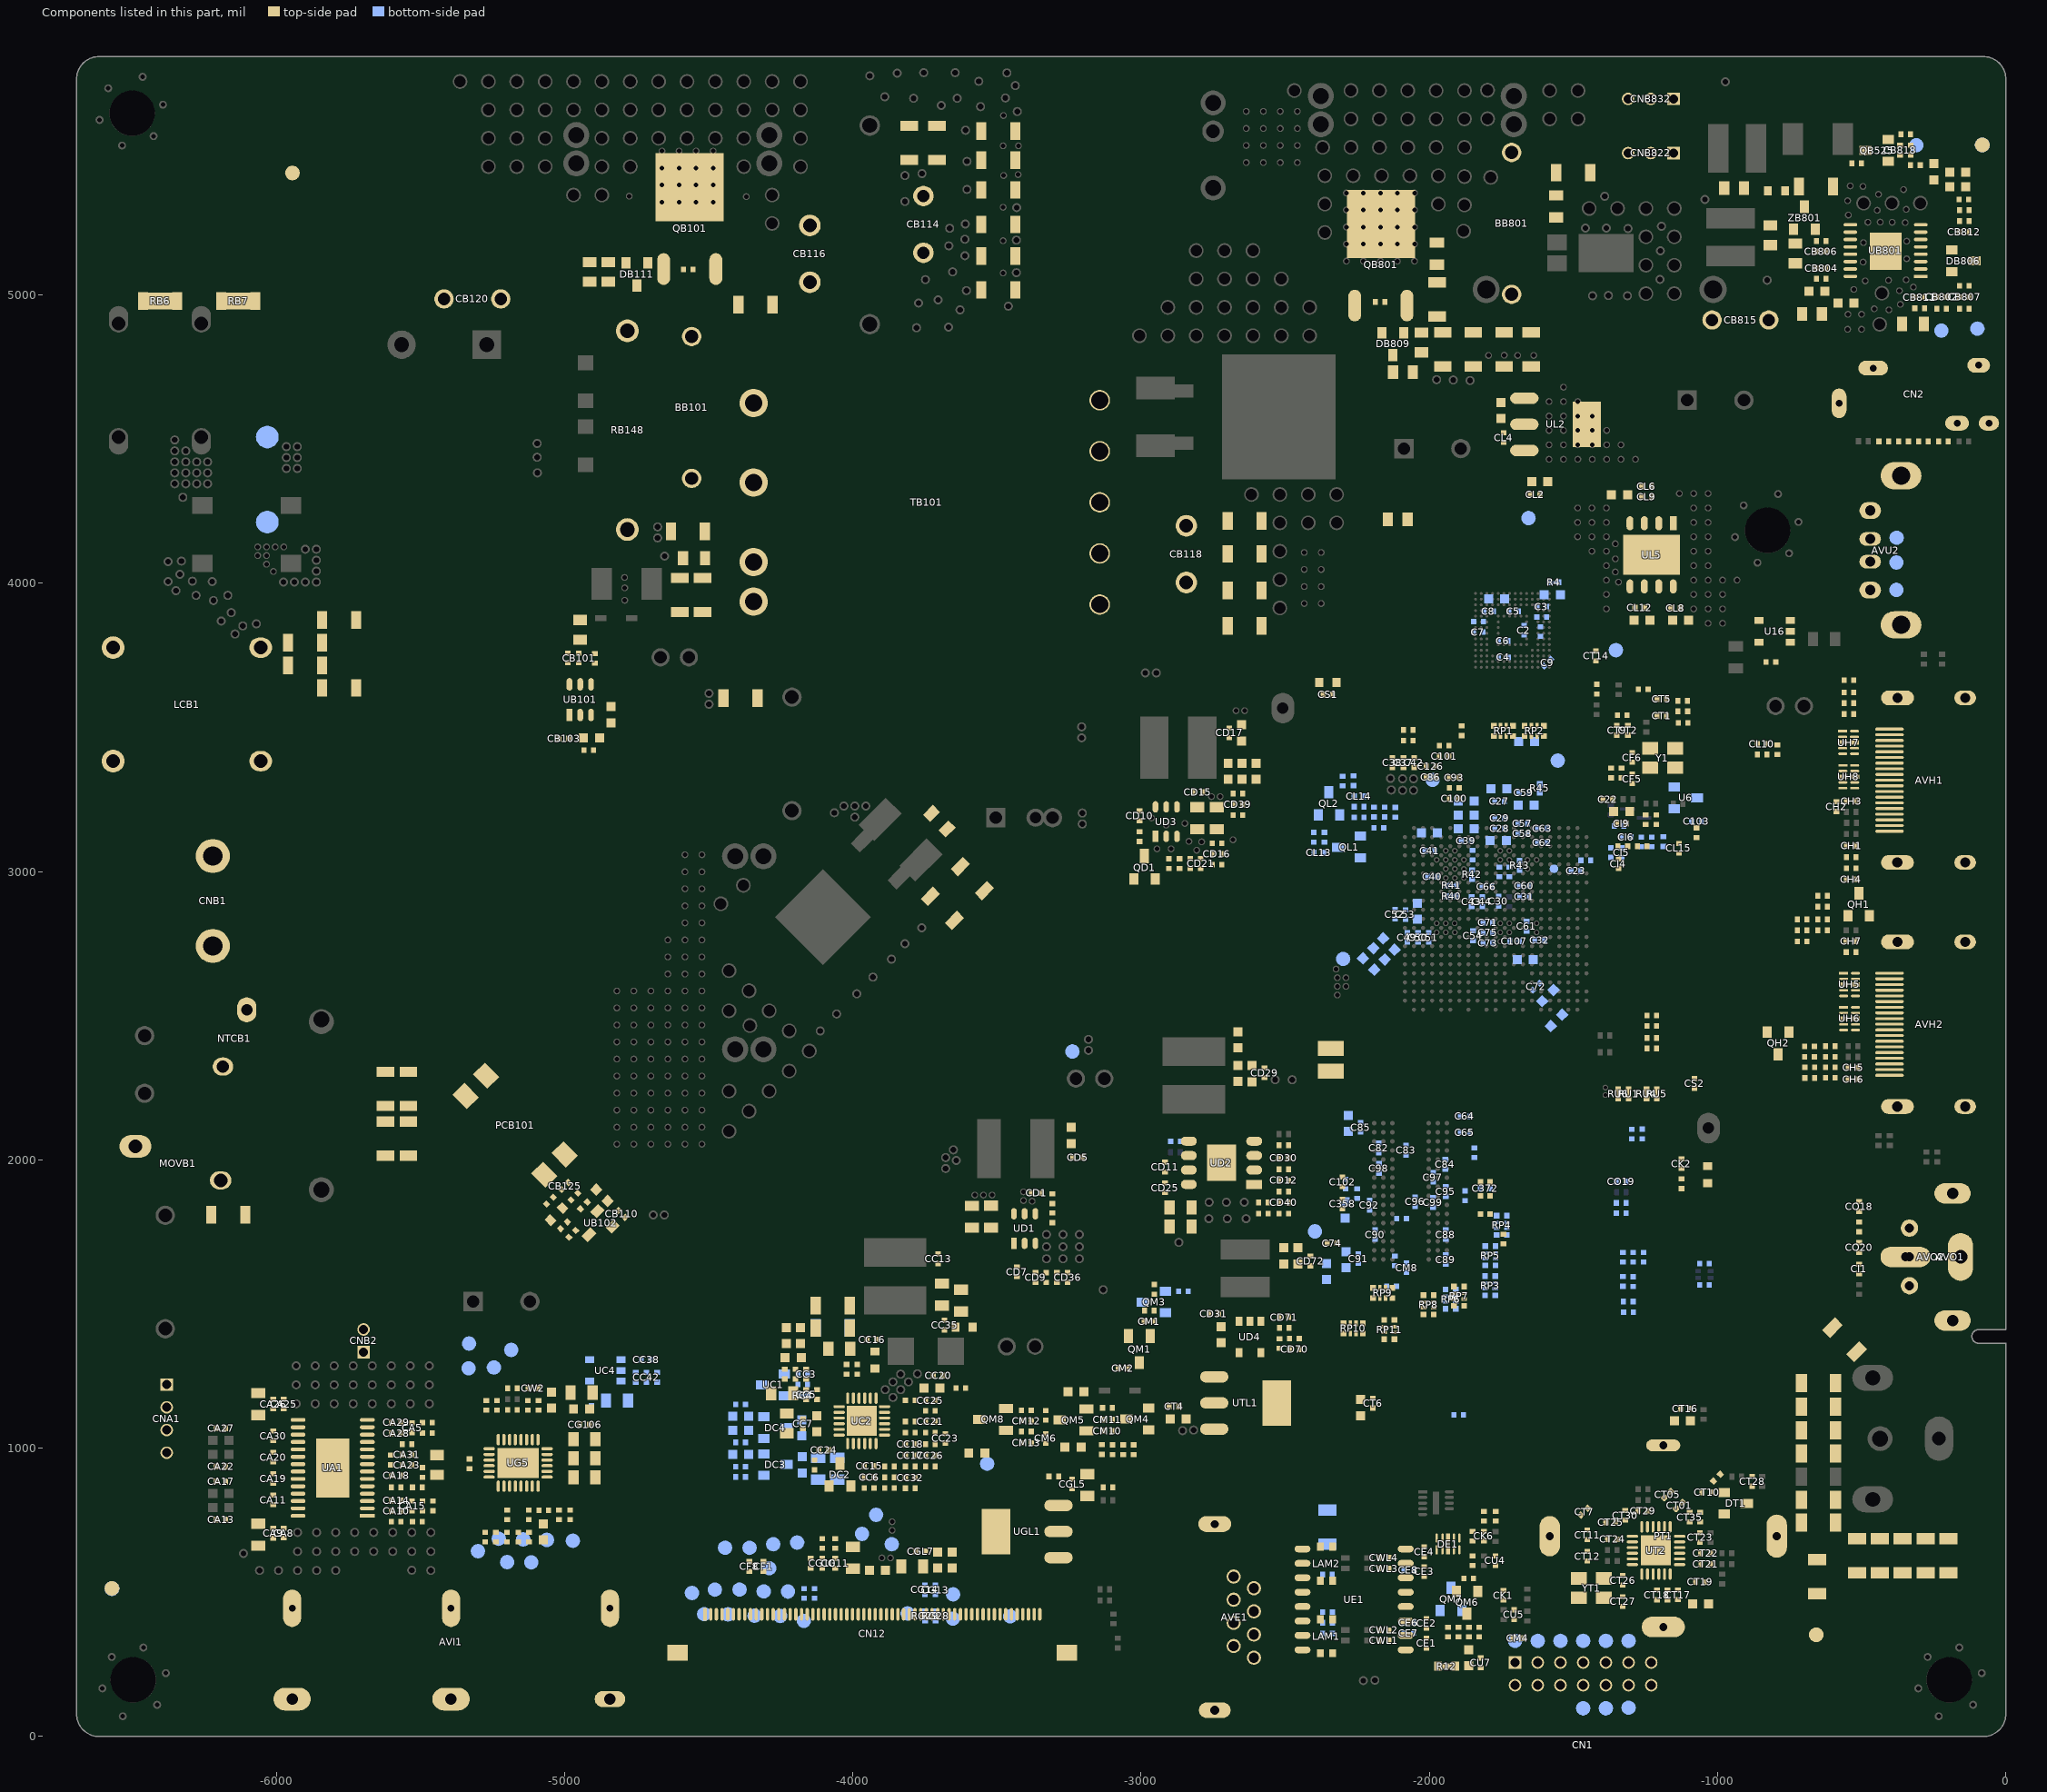
[diagram p0: the components of this part, seen from the top]
# Altium PCB MISC84395.PcbDoc (part 6 of 26)
Units mil, origin at the board's own origin, x right, y up, seen from the top; angles counter-clockwise.
Board outline 6692.91 x 5826.77 mil, 2 copper layers (TopLayer, BottomLayer), stack 61.855 mil thick; 951 components, 565 nets, 4374 pads, 1804 vias.
Unrouted connection lines stored in the file: 1.

## Footprints (in the part's own frame and the unit in brackets; to place one, negate y for a bottom-side part, rotate by r counter-clockwise, add the part's x,y. Pads: shape width x height; smd on the part's side, far side on the other; paste and mask are expansions set on the pad) (continued)
L/LC4/3.2*1.6 [mil] "sunlord,DCM321620F2SF-600T02,17.09.19"
  rect 28x24 smd: 1(59.06,21.65) 2(-59.06,21.65) 3(-59.06,-21.65) 4(59.06,-21.65)
  silkscreen extent -38,-35 99,35, body extent -75,-35 75,35, height 87
L/UU10.5/10*13-2 [mm] "SYUU10.5-L001(协兴电子) 卡扣在侧面"
  oval 1.8x2 hole 1.2: 1(5,-6.5) 4(-5,-6.5)
  round 2 hole 1.2: 2(5,6.5) 3(-5,6.5)
  round 2.2 on Top Overlay: 4(-5,6.5) 4(5,6.5)
  oval 2x2.2 on Top Overlay: 4(-5,-6.5) 4(5,-6.5)
  silkscreen extent -8,-9.25 11.5,9.25, body extent -8,-8.5 9.5,8.5, height 13.8
LB/3.5*6*12.5#1 [mm] "Φ3.5×6.0×0.65mm(编带/秀益达)"
  round 1.7 hole 1.15: 1(-6.25,0) 2(6.25,0)
  round 1.9 on Top Overlay: 35(-6.25,0) 36(6.25,0)
  BottomLayer lines w0.6: 6.185,-0.532 4.05,0 ; -6.185,-0.532 -6.121,-0.516 -4.05,0 ; 6.25,0 4.05,0 ; -6.25,0 -4.05,0 ; 6.185,0.532 4.05,0 ; -6.185,0.532 -6.121,0.516 -5.811,0.439 -4.05,0
  silkscreen extent -5.6,-1.85 5.65,1.85, body extent -6.57,-1.75 6.58,1.75, height 3.5
LB/3.5*6*12.5#2 [mm] "Φ3.5×6.0×0.65mm(编带/秀益达)"
  round 1.7 hole 1.15: 1(-6.25,0) 2(6.25,0)
  round 1.9 on Top Overlay: 35(-6.25,0) 36(6.25,0)
  BottomLayer lines w0.6: 6.185,-0.532 4.05,0 ; -6.185,-0.532 -4.05,0 ; 6.25,0 4.05,0 ; -6.25,0 -4.05,0 ; 6.185,0.532 4.05,0 ; -6.185,0.532 -4.05,0
  silkscreen extent -5.6,-1.85 5.65,1.85, body extent -6.57,-1.75 6.58,1.75, height 3.5
Manufacture_Info [mm]
  round 0.3 on Mech2: 0(0,0)
MARK [mm] "SMD 使用"
  round 1.3 smd paste+0 mask+0.65: 0(0,0)
  TopLayer circle w0.254: c0,0 r1.444
  TopLayer pour cut-out: -1.3,0 -1.201,-0.497 -0.919,-0.919 -0.497,-1.201 0,-1.3 0,-1.3 0.497,-1.201 0.919,-0.919 1.201,-0.497 1.3,0 1.3,0 1.201,0.497 0.919,0.919 0.497,1.201 0,1.3 0,1.3 -0.497,1.201 -0.919,0.919 -1.201,0.497 -1.3,0
Mylar [mil] "180×180×0.4mm-PC-黑色"
NTC(10*5)-V5 [mm] "热敏电阻 SCK152R58MSY  (为勤电子）;161022更新椭圆孔"
  oval 1.6x1.8 hole 1.1: 1(-2.5,1.05)
  oval 1.6x2 on Top Overlay: 2(-2.5,1.05)
  oval 2.2x1.7 hole 1 slot 1.5 at 0 deg: 2(2.5,-1.05)
  oval 2.4x1.9 on Top Overlay: 3(2.5,-1.05)
  silkscreen extent -5.77,-2.5 5.77,2.5, body extent -5.75,-2 5.75,2, height 13.75
OC4-S-1 [mm] "巨路国际；肖特基LTV-817S-TA-B"
  rect 1.5x1.8 smd: 1(-1.27,-4.9) 2(1.27,-4.9) 3(1.27,4.9) 4(-1.27,4.9)
  silkscreen extent -3.17,-5.35 2.55,3.5, body extent -6.95,-6.95 6.95,6.95, height 3.88
OPTICAL-HD-3 [mm] "强生GQ-03-08  通用封装 (TR）  塑胶整体高度11.6mm，中心高度6mm(17.04.28,增加丝印宽度到12.3mm）"
  oval 2x3.4 on Top Overlay: 0(-5.6,4.7) 0(5.6,4.7)
  round 1.778 on Top Overlay: 0(-2.54,8.5) 0(0,8.5) 0(2.54,8.5)
  round 1.524 hole 0.8: 1(-2.54,8.5) 2(0,8.5) 3(2.54,8.5)
  oval 1.8x3.2 hole 1 slot 2.4 at 90 deg: 4(-5.6,4.7) 5(5.6,4.7)
  silkscreen extent -6.15,0 6.15,11.8
PCB_NAME [mm]
  round 0.3 on Mech2: 0(0,0)
PCB_TIME [mm]
  round 0.3 on Mech2: 0(0,0)
PHONE-HD-54 [mm] "CS,PJ-304L-EP(706-0003-0661),中心高度2.5mm，19.03.15"
  oval 1.5x2.3 on Top Overlay: 0(-2.55,4.3)
  oval 1.5x2 on Top Overlay: 0(-2.55,1.5)
  oval 2.8x1.5 on Top Overlay: 0(-0.8,14.7)
  round 1.8 on Keep-Out: 0(0,10.5) 0(0,3.5)
  oval 1.5x2.8 on Top Overlay: 0(2.3,11.7)
  oval 1.5x2.2 on Top Overlay: 0(2.55,2.4)
  oval 1.3x2 hole 0.6 slot 1.3 at 90 deg: 1(2.55,2.4)
  oval 1.3x2.6 hole 0.6 slot 1.9 at 90 deg: 2(2.3,11.7)
  oval 1.3x2.1 hole 0.6 slot 1.4 at 90 deg: 3(-2.55,4.3)
  oval 2.6x1.3 hole 0.6 slot 1.9 at 0 deg: 4(-0.8,14.7)
  oval 1.3x1.8 hole 0.6 slot 1.1 at 90 deg: 5(-2.55,1.5)
  silkscreen extent -3.1,0 3.1,14.95, body extent -3,-2.5 3,14.85, height 5
QFN24/0.5-1 [mm] "MxL601(MAXLINEAR)"
  oval 1x0.26 smd: 1(-2.08,1.25) 2(-2.08,0.75) 3(-2.08,0.25) 4(-2.08,-0.25) 5(-2.08,-0.75) 6(-2.08,-1.25) 13(2.08,-1.25) 14(2.08,-0.75) 15(2.08,-0.25) 16(2.08,0.25) 17(2.08,0.75) 18(2.08,1.25)
  oval 0.26x1 smd: 7(-1.25,-2.08) 8(-0.75,-2.08) 9(-0.25,-2.08) 10(0.25,-2.08) 11(0.75,-2.08) 12(1.25,-2.08) 19(1.25,2.08) 20(0.75,2.08) 21(0.25,2.08) 22(-0.25,2.08) 23(-0.75,2.08) 24(-1.25,2.08)
  rect 2.65x2.65 smd paste-0.6 mask-0.6: 25(0,0)
  TopLayer pour cut-out: -2.08,1.25 -2.08,-1.25 -1.25,-2.08 1.25,-2.08 2.08,-1.25 2.08,1.25 1.25,2.08 -1.25,2.08
  silkscreen extent -3.31,-3.51 3.31,3.46, body extent -2.02,-2.02 2.02,2.02, height 1
QFN24/0.5-5 [mm] "BEKEN ,     BK2433;BQ24196(1mm)"
  oval 1x0.27 smd: 1(-2,1.25) 2(-2,0.75) 3(-2,0.25) 4(-2,-0.25) 5(-2,-0.75) 6(-2,-1.25) 13(2,-1.25) 14(2,-0.75) 15(2,-0.25) 16(2,0.25) 17(2,0.75) 18(2,1.25)
  oval 0.27x1 smd: 7(-1.25,-2) 8(-0.75,-2) 9(-0.25,-2) 10(0.25,-2) 11(0.75,-2) 12(1.25,-2) 19(1.25,2) 20(0.75,2) 21(0.25,2) 22(-0.25,2) 23(-0.75,2) 24(-1.25,2)
  rect 2.667x2.667 smd paste-0.6 mask-0.6: 25(0,0)
  silkscreen extent -3.38,-3.5 3.1,3.5, body extent -2.05,-2.05 2.05,2.05, height 1
QFN28/0.5-5 [mm] "RICHTEK,RT8939GQW,16.12.16"
  oval 1x0.28 smd: 1(-2.05,1.75) 2(-2.05,1.25) 3(-2.05,0.75) 4(-2.05,0.25) 5(-2.05,-0.25) 6(-2.05,-0.75) 7(-2.05,-1.25) 8(-2.05,-1.75) 15(2.05,-1.75) 16(2.05,-1.25) 17(2.05,-0.75) 18(2.05,-0.25) 19(2.05,0.25) 20(2.05,0.75) 21(2.05,1.25) 22(2.05,1.75)
  oct 1x1 on Top Solder paste-0.1 mask+0.102: 2(-0.66,1.25) 2(-0.66,-1.25) 2(-0.66,0) 3(0.66,1.25) 3(0.66,-1.25) 3(0.66,0)
  oct 1x1 on Top Paste paste-0.1 mask+0.102: 2(-0.66,1.25) 2(-0.66,-1.25) 2(-0.66,0) 3(0.66,1.25) 3(0.66,-1.25) 3(0.66,0)
  oval 0.28x1 smd: 9(-1.25,-2.55) 10(-0.75,-2.55) 11(-0.25,-2.55) 12(0.25,-2.55) 13(0.75,-2.55) 14(1.25,-2.55) 23(1.25,2.55) 24(0.75,2.55) 25(0.25,2.55) 26(-0.25,2.55) 27(-0.75,2.55) 28(-1.25,2.55)
  rect 2.65x3.65 smd paste-3 mask-3: EPAD(0,0)
  silkscreen extent -3.63,-3.93 3.43,3.7, body extent -2.05,-2.55 2.05,2.55, height 0.8
R2-H-17.5 [mm] "只适用于2W小型化"
  round 2 hole 1.3: 1(-8.75,0) 2(8.75,0)
  round 2.2 on Top Overlay: 69(-8.75,0) 69(8.75,0)
  BottomLayer lines w0.6: 8.654,0.643 8.562,0.615 6.55,0 ; -8.665,0.606 -8.583,0.583 ; -8.75,0 -8.634,0 -6.55,0 ; 8.75,0 6.55,0 ; 8.665,-0.606 8.583,-0.583 ; -8.654,-0.643 -8.562,-0.615 -6.55,0 ; -8.583,0.583 -8.583,0.583 ; -8.583,0.583 -6.55,0 ; 6.55,0 8.583,-0.583 ; 8.583,-0.583 8.583,-0.583 ; 8.583,-0.583 8.583,-0.583 ; 8.583,-0.583 8.583,-0.583
  silkscreen extent -8,-2.25 8.1,2.25, body extent -9.14,-2.25 9.14,2.25, height 4.5
R0402 [mm] "片式电阻"
  rect 0.45x0.5 smd mask+0.076: 1(-0.425,0) 2(0.425,0)
  silkscreen extent -0.8,-0.4 0.8,0.4, body extent -0.5,-0.25 0.5,0.25, height 0.5
R0402SC#1 [mm]
  rect 0.45x0.5 smd mask+0.076: 1(-0.425,0) 2(0.425,0)
  rect 0.42x0.25 smd paste-0.5 mask-0.5: 3(0,0)
  silkscreen extent -0.8,-0.4 0.8,0.4, body extent -0.5,-0.25 0.5,0.25, height 0.5
R0402SC#2 [mm]
  rect 0.45x0.5 smd mask+0.076: 1(-0.425,0) 2(0.425,0)
  rect 0.42x0.457 smd paste-0.5 mask-0.5: 3(0,0)
  silkscreen extent -0.8,-0.4 0.8,0.4, body extent -0.5,-0.25 0.5,0.25, height 0.5
R0603 [mm] "贴片电阻"
  rect 0.7x0.8 smd mask+0.076: 1(-0.756,0) 2(0.756,0)
  silkscreen extent -1.25,-0.54 1.25,0.54, body extent -0.8,-0.4 0.8,0.4, height 0.8
R0603SC [mm] "贴片电阻"
  rect 0.7x0.8 smd mask+0.076: 1(-0.756,0) 2(0.756,0)
  rect 0.82x0.5 smd paste-0.5 mask-0.5: 3(0,0)
  silkscreen extent -1.25,-0.54 1.25,0.54, body extent -0.8,-0.4 0.8,0.4, height 0.8
R0805 [mm] "贴片电阻"
  rect 0.9x1.2 smd mask+0.076: 1(-0.866,0) 2(0.866,0)
  silkscreen extent -1.47,-0.75 1.47,0.75, body extent -1,-0.62 1,0.63, height 0.5
R1206 [mm] "贴片电阻"
  rect 0.9x1.55 smd mask+0.076: 1(-1.5,0) 2(1.5,0)
  silkscreen extent -2.1,-0.93 2.1,0.93, body extent -1.6,-0.8 1.6,0.8, height 0.55
R1206SC [mm] "贴片电阻"
  rect 0.9x1.55 smd mask+0.076: 1(-1.5,0) 2(1.5,0)
  rect 2.7x1.5 smd paste-2.7 mask-2.7: 3(0,0)
  silkscreen extent -2.1,-0.93 2.1,0.93, body extent -1.6,-0.8 1.6,0.8, height 0.55
RA0402 [mm] "排阻"
  rect 0.5x0.5 smd mask+0.076: 1(-0.45,0.85) 2(0.45,0.85) 7(-0.45,-0.85) 8(0.45,-0.85)
  rect 0.5x0.3 smd mask+0.076: 3(-0.45,0.25) 4(0.45,0.25) 5(-0.45,-0.25) 6(0.45,-0.25)
  silkscreen extent -0.85,-1.27 0.85,1.27, body extent -0.51,-1 0.51,1, height 0.35
RCL0524P [mm] "RCLAMP0524J(19.03.04 优化丝印）"
  rect 0.21x0.8 smd: 1(-1,-0.52)
  oval 0.21x0.8 smd: 2(-0.5,-0.52) 3(0.5,-0.52) 4(1,-0.52) 5(1,0.52) 6(0.5,0.52) 7(-0.5,0.52) 8(-1,0.52)
  rect 0.38x0.8 smd: GND(0,-0.52) GND(0,0.52)
  silkscreen extent -1.4,-2.03 1.4,1.14, body extent -1.25,-0.6 1.25,0.6, height 0.66
RJ45-VD-16 [mm] "YUQIU,RJ170-F08M1BY-B,19.03.16"
  oval 1.6x3.1 on Top Overlay: 0(-8.2,-1.5) 0(8.2,-1.5)
  round 1.45 on Top Overlay: 0(-3.57,-4.95) 0(-2.55,-3.17) 0(-1.53,-4.95) 0(-0.51,-3.17) 0(0.51,-4.95) 0(1.53,-3.17) 0(2.55,-4.95) 0(3.57,-3.17)
  round 1.25 hole 0.9: 1(3.57,-3.17) 2(2.55,-4.95) 3(1.53,-3.17) 4(0.51,-4.95) 5(-0.51,-3.17) 6(-1.53,-4.95) 7(-2.55,-3.17) 8(-3.57,-4.95)
  oval 1.4x2.8 hole 0.8 slot 2.2 at 90 deg: 9(-8.2,-1.5)
  oval 1.4x2.9 hole 0.7 slot 2.2 at 90 deg: 10(8.2,-1.5)
  silkscreen extent -9.05,-5.93 9.05,5.94, body extent -8.85,-5.77 8.85,5.78, height 13
SHIELD(16*20*6) [mm] "屏蔽罩：用于与高频头分离的做法"
  oval 2.1x4.1 on Top Overlay: 0(-8,10) 0(8,10)
  oval 4.1x2.1 on Top Overlay: 0(0,20) 0(0,0)
  oval 3.8x1.8 hole 0.7 slot 2.7 at 0 deg: 1(0,0)
  oval 1.038x3.013 / inner oval 1.8x3.8 / far side oval 1.8x3.8 hole 0.7 slot 2.7 at 90 deg: 2(8,10)
  oval 3.556x1.8 hole 0.7 slot 2.7 at 0 deg: 3(0,20)
  oval 1.8x3.8 hole 0.7 slot 2.7 at 90 deg: 4(-8,10)
  silkscreen extent -9,-1 9,21, body extent -8.57,-0.15 8.57,20.15, height 6
"Silica gel(3*2*2.5)" [mm] "导电硅胶,3×2×2.5mm;15.09.17"
  rect 1.3x2.3 smd: 1(-1,0) 2(1,0)
  silkscreen extent -1.9,-1.4 1.9,1.4
"Silica gel-10" [mil] "硅胶"
  silkscreen extent -118,-197 118,197
"Silica gel-15" [mil] "硅胶"
  silkscreen extent -118,-295 118,295
SIP2*7H/2.0DM-8 [mm] "XFE,JN-2.0-2×7PW-H=5.6-PC=2.5,公座，19.03.13"
  round 0.8 on Mech2: 0(-6,-3.625) 0(-4,-3.625) 0(-4,-5.625) 0(-2,-3.625) 0(-2,-5.625) 0(0,-3.625) 0(0,-5.625) 0(2,-3.625) 0(2,-5.625) 0(4,-3.625) 0(4,-5.625) 0(6,-3.625) 0(6,-5.625)
  rect 0.8x0.8 on Mech2: 0(-6,-5.625)
  rect 1.3x1.3 on Top Overlay: 0(-6,8.876)
  round 1.3 on Top Overlay: 0(-6,6.876) 0(-4,8.876) 0(-4,6.876) 0(-2,8.876) 0(-2,6.876) 0(0,8.876) 0(0,6.876) 0(2,8.876) 0(2,6.876) 0(4,8.876) 0(4,6.876) 0(6,8.876) 0(6,6.876)
  rect 1.1x1.1 hole 0.8: 1(-6,8.876)
  round 1.1 hole 0.8: 2(-6,6.876) 3(-4,8.876) 4(-4,6.876) 5(-2,8.876) 6(-2,6.876) 7(0,8.876) 8(0,6.876) 9(2,8.876) 10(2,6.876) 11(4,8.876) 12(4,6.876) 13(6,8.876) 14(6,6.876)
  silkscreen extent -8.5,0 8.13,10.29
SIP2/2.0D-1 [mm] "捷仕泰/铭锋达"
  rect 1.3x1.3 on Top Overlay: 0(-1,0)
  round 1.3 on Top Overlay: 0(1,0)
  rect 1.1x1.1 hole 0.8: 1(-1,0)
  round 1.1 hole 0.8: 2(1,0)
  silkscreen extent -3,-3.2 3,1.8, body extent -3,-3.2 3,1.8, height 6
SIP3/2.0D-CP [mm] "捷仕泰/铭锋达;带扣插座与非带扣插座 兼容；15.07.11"
  rect 1.4x1.4 on Top Overlay: 0(-2,0)
  round 1.4 on Top Overlay: 0(0,0) 0(2,0)
  rect 1.1x1.1 hole 0.8: 1(-2,0)
  round 1.1 hole 0.8: 2(0,0) 3(2,0)
  silkscreen extent -4,-3.2 4,3.07, body extent -4,-3.2 4,1.8, height 6
SIP3H/2.0D-3 [mm] "捷仕泰：A2004AW-03-A1MA-P，带扣，加强筋"
  rect 1.6x1.6 on Top Overlay: 0(-2,0)
  round 1.6 on Top Overlay: 0(0,0) 0(2,0)
  rect 1.1x1.1 hole 0.8: 1(-2,0)
  round 1.1 hole 0.8: 2(0,0) 3(2,0)
  silkscreen extent -4.1,-7.95 4.1,1.5
SIP4H/2.0D-6 [mm] "捷仕泰：A2004AWD-04-A1MA-P"
  rect 1.6x1.6 on Top Overlay: 0(-3,0)
  round 1.6 on Top Overlay: 0(-1,0) 0(1,0) 0(3,0)
  rect 1.1x1.1 hole 0.8: 1(-3,0)
  round 1.1 hole 0.8: 2(-1,0) 3(1,0) 4(3,0)
  silkscreen extent -5.1,-7.95 5.1,1.5, body extent -5,-8 5,1.2, height 5.1
SO-23 [mm] "双向二极管封装"
  rect 0.8x1 smd: 1(0.953,1.016) 3(-0.953,1.016)
  rect 0.8x1.1 smd: 2(0,-0.966)
  silkscreen extent -1.55,-0.86 1.55,0.36, body extent -1.5,-1.25 1.5,1.25, height 1.1
SO-23-1 [mm] "双向二极管封装，小型"
  rect 0.8x1 smd: 1(-0.953,-1.016) 2(0.953,-1.016)
  rect 0.8x1.1 smd: 3(0,0.966)
  silkscreen extent -1.55,-0.36 1.55,0.86, body extent -1.5,-1.25 1.5,1.25, height 1.1
SOP8/1.27 [mm] "LOW POWER SEMI;LP28009(18.12.20 增大焊盘内延）"
  rect 1.4x0.8 smd: 1(-2.88,1.905)
  oval 1.4x0.8 smd: 2(-2.88,0.635) 3(-2.88,-0.635) 4(-2.88,-1.905) 5(2.88,-1.905) 6(2.88,-0.635) 7(2.88,0.635) 8(2.88,1.905)
  rect 2.55x3.2 smd paste-3 mask-3: 9(0,0)
  silkscreen extent -4.7,-2.5 4.16,2.5, body extent -3.1,-2.5 3.1,2.5, height 1.76
SOP8/1.27-3 [mm] "LEADCHIP;LC1118;14-05-09"
  rect 1.238x0.6 smd: 1(-2.783,1.905)
  oval 1.238x0.6 smd: 2(-2.782,0.635) 3(-2.782,-0.635) 4(-2.783,-1.905) 5(2.783,-1.905) 6(2.783,-0.635) 7(2.783,0.635) 8(2.783,1.905)
  rect 3.5x5 smd paste-3 mask-3: EPAD(0,0)
  silkscreen extent -4.65,-2.5 4.16,2.5, body extent -3.1,-2.5 3.1,2.5, height 1.76
SOP16/1.27-2 [mm] "Pulse, H1260NL H16101MC-C"
  oval 1.4x0.6 smd: 1(-4.55,4.445) 2(-4.55,3.175) 3(-4.55,1.905) 4(-4.55,0.635) 5(-4.55,-0.635) 6(-4.55,-1.905) 7(-4.55,-3.175) 8(-4.55,-4.445) 9(4.55,-4.445) 10(4.55,-3.175) 11(4.55,-1.905) 12(4.55,-0.635) 13(4.55,0.635) 14(4.55,1.905) 15(4.55,3.175) 16(4.55,4.445)
  silkscreen extent -5.8,-6.35 6.2,6.35, body extent -3.72,-6.35 3.72,6.35, height 6
SOP28/0.65-7 [mm] "ESMT,AD52050B-26QG28NRR,0723_2018"
  oct 1.2x1 on Top Solder mask+0: 0(-0.75,1.95) 0(-0.75,0.65) 0(-0.75,-0.65) 0(-0.75,-1.95) 0(0.75,1.95) 0(0.75,0.65) 0(0.75,-0.65) 0(0.75,-1.95)
  oct 1.2x1 on Top Paste mask+0: 0(-0.75,1.95) 0(-0.75,0.65) 0(-0.75,-0.65) 0(-0.75,-1.95) 0(0.75,1.95) 0(0.75,0.65) 0(0.75,-0.65) 0(0.75,-1.95)
  rect 1.3x0.35 smd mask+0.051: 1(-3.05,4.225)
  oval 1.3x0.35 smd mask+0.051: 2(-3.05,3.575) 3(-3.05,2.925) 4(-3.05,2.275) 5(-3.05,1.625) 6(-3.05,0.975) 7(-3.05,0.325) 8(-3.05,-0.325) 9(-3.05,-0.975) 10(-3.05,-1.625) 11(-3.05,-2.275) 12(-3.05,-2.925) 13(-3.05,-3.575) 14(-3.05,-4.225) 15(3.05,-4.225) 16(3.05,-3.575) 17(3.05,-2.925) 18(3.05,-2.275) 19(3.05,-1.625) 20(3.05,-0.975) 21(3.05,-0.325) 22(3.05,0.325) 23(3.05,0.975) 24(3.05,1.625) 25(3.05,2.275) 26(3.05,2.925) 27(3.05,3.575) 28(3.05,4.225)
  rect 2.9x5.2 smd paste-5 mask-5: EPAD(0,0)
  silkscreen extent -4.68,-4.9 4.44,4.9, body extent -3.2,-4.9 3.2,4.9, height 1.2
SOT-23 [mm]
  rect 0.8x1 smd: B(0.952,1.016) E(-0.953,1.016)
  rect 0.8x1.1 smd: C(-0.013,-0.966)
  silkscreen extent -1.55,-0.81 1.55,0.36, body extent -1.5,-1.25 1.5,1.25, height 1.1
SOT-23-1 [mm]
  rect 0.8x1.1 smd: D(0,-1.15)
  rect 0.8x1.27 smd: G(0.95,1.2) S(-0.95,1.2)
  TopLayer pour cut-out: -1.583,0.903 -1.583,-0.905 1.587,-0.905 1.587,0.903
  silkscreen extent -1.55,-1.05 1.55,0.33, body extent -1.52,-1.48 1.52,1.48, height 1.25
SOT-23-5 [mm] "LPW5206(1.295mm)"
  rect 0.6x0.8 smd: 1(-0.95,-1.375) 2(0,-1.375) 3(0.95,-1.375) 4(0.95,1.375) 5(-0.95,1.375)
  silkscreen extent -1.5,-2.49 1.5,0.85, body extent -1.5,-0.85 1.5,0.85, height 1.45
SOT-23-7 [mil] "对应2N7002 MOS管，大小和SOT-23一样"
  rect 31.5x50 smd: D(0,40)
  rect 31.5x39.37 smd: G(-37.5,-40) S(37.5,-40)
  TopLayer pour cut-out: 64.07,-39.32 64.07,36.28 -60.76,36.28 -60.76,-39.32
  silkscreen extent -60,-14 60,34, body extent -59,-49 59,49, height 43
SOT-23-RAK [mm] "TL431G-AE2-R(UTC)"
  rect 0.8x1.1 smd: A(0.013,0.966)
  rect 0.8x1 smd: K(0.953,-1.016) R(-0.952,-1.016)
  silkscreen extent -1.52,-0.36 1.52,0.86, body extent -1.5,-1.25 1.5,1.25, height 1.1
SOT-26 [mm] "LD7536R"
  rect 0.5x1.1 smd: 1(0.95,1.35)
  oval 0.5x1.1 smd: 2(0,1.35) 3(-0.95,1.35) 4(-0.95,-1.35) 5(0,-1.35) 6(0.95,-1.35)
  silkscreen extent -1.55,-2.54 1.55,2.9, body extent -1.55,-0.9 1.55,0.9, height 1.45
SOT-223 [mm]
  oval 1x2.5 smd: 1(-2.3,-2.75) 2(0,-2.75) 3(2.3,-2.75)
  rect 4x2.5 smd: 4(0,2.75)
  TopLayer pour cut-out: 2.3,-1.188 2.3,-4.312 -2.345,-4.312 -2.64,-4.253 -2.891,-4.086 -3.058,-3.835 -3.117,-3.54 -3.117,-3.54 -2.299,-3.54 -2.299,-1.956 -3.124,-1.956 -3.066,-1.662 -2.899,-1.413 -2.65,-1.247 -2.356,-1.188 -2.356,-1.188
  silkscreen extent -3.45,-2.75 3.45,2.81, body extent -3.35,-3.3 3.35,3.4, height 1.7
T/EQ2512*11 [mm] "14.05.20修改外形，磁芯大小，增加胶纸尺寸,20180130修改焊盘大小满足磁芯的安规距离,增加开槽标示。"
  round 2.5 hole 1.5 mask+0.076: 1(-12.55,8.75) 3(-12.55,1.75) 5(-12.55,-5.25) 6(-12.55,-8.75)
  round 2.7 on Top Overlay mask+0.076: 2(-12.55,8.75) 3(-12.55,1.75) 6(-12.55,-5.25) 7(-12.55,-8.75)
  round 1.8 / inner round 1.8 / far side round 2.5 hole 1.5 mask+0.076: 7(17.95,-9) 8(17.95,-4.5) 9(17.95,0) 10(17.95,4.5) 11(17.95,9)
  round 2 on Top Overlay mask+0.076: 12(17.95,-9) 12(17.95,-4.5) 12(17.95,0) 12(17.95,4.5) 12(17.95,9)
  silkscreen extent -15.55,-14 20.98,14
TO-252-GDS [mm] "SC08440  IRLR024N"
  rect 6x6 smd: D(0,0)
  oval 1.143x2.794 smd: G(-2.3,-7.2) S(2.3,-7.2)
  silkscreen extent -3.4,-5.64 3.4,3.4, body extent -3.4,-7.75 3.4,2.45, height 2.5
TP#1 [mil] "TEST POINT"
  round 50 smd: 1(0,0)
TP#2 [mil] "TEST POINT"
  round 50 smd paste-50: 1(0,0)
TP#3 [mil] "TEST POINT"
  round 30 smd: 1(0,0)
TP-TDT [mm] "电源放电测试点，间隔7.5mm"
  round 2 smd paste-2: 1(-3.75,0) 2(3.75,0)
  silkscreen extent -5.75,-2 5.75,2
TP_BL [mil] "TEST POINT,专用背光测试点"
  round 50 smd paste-50: 1(0,0)
  silkscreen extent -252,-38 37,38
TSOT23-6 [mm] "MP65151DJ[MPS]/MP1470"
  rect 1x0.5 smd: 1(-1.3,0.95)
  oval 1x0.5 smd: 2(-1.3,0) 3(-1.3,-0.95) 4(1.3,-0.95) 5(1.3,0) 6(1.3,0.95)
  silkscreen extent -2.92,-1.5 0.85,1.5, body extent -0.85,-1.5 0.85,1.5, height 1
TSSOP16/0.65-3 [mm] "LINEAR;LTC3413"
  rect 0.95x1.2 on Top Solder: 0(-0.625,0.75) 0(-0.625,-0.75) 0(0.625,-0.75) 0(0.625,0.75)
  rect 0.95x1.2 on Top Paste: 0(-0.625,0.75) 0(-0.625,-0.75) 0(0.625,-0.75) 0(0.625,0.75)
  rect 1.2x0.3 smd: 1(-3.1,2.213)
  oval 1.2x0.3 smd: 2(-3.1,1.563) 3(-3.1,0.913) 4(-3.1,0.263) 5(-3.1,-0.387) 6(-3.1,-1.037) 7(-3.1,-1.687) 8(-3.1,-2.337) 9(3.1,-2.338) 10(3.1,-1.687) 11(3.1,-1.038) 12(3.1,-0.387) 13(3.1,0.262) 14(3.1,0.913) 15(3.1,1.562) 16(3.1,2.213)
  rect 2.8x3.3 smd paste-5 mask-5: 17(0,0)
  silkscreen extent -4.93,-2.55 4.55,2.67, body extent -3.2,-2.61 3.2,2.55, height 1.1
USB1-HD-2 [mm] "捷仕泰 ： U2504M-04-E1WD-C；170204加宽后壳丝印(18.03.12,更新信号脚孔径）"
  oval 2.7x3.9 on Top Overlay: 0(-6.57,10.257) 0(6.57,10.247)
  oval 1.7x2.1 on Top Overlay: 0(-3.5,12.957) 0(3.5,12.957)
  oval 1.5x1.9 hole 0.9 slot 1.4 at 90 deg: 1(-3.5,12.957) 4(3.5,12.957)
  oval 1.4x2.1 on Top Overlay: 1(-1,12.957) 2(1,12.957)
  oval 1.2x1.9 hole 0.9 slot 1.4 at 90 deg: 2(-1,12.957) 3(1,12.957)
  oval 2.4x3.6 / inner oval 2.4x3.6 / far side oval 2.8x4 hole 1.6 slot 2.3 at 90 deg: 5(6.57,10.247) 6(-6.57,10.247)
  TopLayer pour cut-out: 2.433,14.667 4.428,14.667 4.532,14.647 4.62,14.588 4.678,14.5 4.699,14.396 4.699,14.396 4.699,11.335 4.68,11.238 4.625,11.156 4.542,11.101 4.445,11.081 4.445,11.081 2.422,11.081 2.422,14.656
  KeepOutLayer pour cut-out: -3.49,14.696 -4.146,14.566 -4.703,14.194 -5.075,13.637 -5.206,12.98 -5.206,12.98 -5.206,12.94 -5.068,12.25 -4.677,11.665 -4.092,11.275 -3.402,11.137 -3.402,11.137 2.42,11.137 2.637,11.18 2.821,11.303 2.943,11.487 2.986,11.703 2.986,11.703 2.986,14.149 2.944,14.361 2.824,14.541 2.644,14.661 2.432,14.704 2.432,14.704 -3.482,14.704 -3.485,14.703 -3.487,14.701 -3.489,14.699 -3.49,14.696
  silkscreen extent -7.1,2.04 7.05,14.58, body extent -10,-87.25 10,14.14, height 8.2
VR(13*5)-V-7.5 [mm] "为勤,VARISTOR,17.01.04修改为椭圆孔;160105更新椭圆孔"
  oval 2.8x2 hole 1.2 slot 2 at 0 deg: 1(3.75,-1.5)
  oval 1.9x1.6 hole 1.2: 2(-3.75,1.5)
  oval 2.1x1.8 on Top Overlay: 2(-3.75,1.5)
  oval 3x2.2 on Top Overlay: 2(3.75,-1.5)
  silkscreen extent -6.65,-2.5 6.42,2.5, body extent -6.5,-2.75 6.5,2.75, height 15.5
XTAL-S-3 [mm] "三星（SQ3D03200D2IBA）晶振"
  rect 1.4x1.1 smd: 1(-1.1,-0.85) 2(1.1,-0.85) 3(1.1,0.85) 4(-1.1,0.85)
  silkscreen extent -2.37,-1.91 1.65,1.3, body extent -1.65,-1.3 1.65,1.3, height 0.8

## Part data
ADIM BL_ON PWM_DIM: library part TEST
AVE1: library part XXX.XXX.0004736-DHMI, "Network terminal,DIP,RJ170-F08M1BY-B,YUQIU-DHMI"
AVH1 AVH2: library part HHF-14B000-2SA-H-D-HDMI, "CN-HDMI-horizontal-#-#"
AVI1: library part XXX.XXX.0001407-DHMI, "RCA terminal,RCA Jack,AV3,V,Yellow, White, Red,D14,DIP,CYB-3.2-3DL11-1-100(R),YK-DHMI"
AVO1: library part XXX.XXX.0000032-DLMI, "RCA terminal,RCA Jack,AV1,H,Orange,CH6.5,Seal,DIP,AV19-01S-0020,QS-DLMI"
AVO2: library part XXX.XXX.0001777-DLMI, "Optical fiber terminal,OPTICAL,H,DIP,182500191,VAST-DLMI"
AVU2: library part USB-2035A01-DHMI-USB, "CN-USB-#-#-#"
BB101: library part φ3.5×6.0×0.65mm-CP(编带/秀益达)-DAI, "Through-hole ferrite bead"
BB801: library part φ3.5×6.0×0.65mm-CP(编带/秀益达)-DLAI, "Through-hole ferrite bead"
C1 C21 C25 C26 C33 C34 C35 C36 C45 C46 C47 C48 C55 C56 C80 C81 C87 C94 C104 C105 C106 C108 CD2 CD8 CD26 CD28 CD69 CD73 CD74 CGL6 CGL49 CL1 CL3 CL5 CL7 CL11 CM3 CM7 CM9 CT3 CT8 CT15 CT50 CU6: library part 10uF-0603-X5R-±20%-6.3V-D
C2 C5 C44 C54 C60 C62 C74 C75 C85 C92 C99 CC6 CC7 CC15 CC17 CC18 CH2 CT17 CT25 CT30: library part 1uF-0402-X5R-±20%-6.3V-D
C3 C4 C6 C7 C8 C22 C32 C61 C66 C103 C372 CA10 CA14 CA28 CA29 CC23 CC24 CC42 CD1 CD5 CD11 CD15 CD17 CD25 CD29 CD39 CD40 CE6 CE8 CG10 CG11 CG13 CG14 CG106 CI1 CL2 CL4 CM1 CM2 CU7 CW2 CWL1 CWL2 CWL3 CWL4: library part 0.1uF-0402-X5R-±20%-16V-D
C9 C64 C65: library part 2.2uF-0402-X5R-±20%-6.3V-D
C23 CI4: library part 0.047uF-0402-X7R-±10%-16V-D
C27 C28 C29 C30 C31 C37 C38 C39 C40 C41 C42 C43 C49 C50 C51 C52 C53 C57 C58 C59 C63 C71 C72 C73 C82 C83 C84 C88 C89 C90 C91 C95 C96 C97 C98 C100 C107 C126 C358 CD31 CGL5 CGL7 CL6 CL8 CL9 CL12: library part 0.1uF-0402-X7R-±10%-16V-D
C86 CK1 CK2 CM4 CM8 CT18 CU4 CU5: library part 0.01uF-0402-X7R-±10%-50V-D
C93 CE7: library part 0.01uF-0402-X7R-±10%-16V-D
C101 C102 CA9 CA26 CB103 CH1 CH4 CH5 CH6 CS1 CS2 CT21 CT22 CT28: library part 1000pF-0402-X7R-±10%-50V-D
CA1 CA2 CC8 CC12 CC29 CC30 CC43 CD4 CD6 CD13 CD14 CD23 CD24 CG1 CG2 CG3 CG104 CGL4: library part 10uF-0805-X5R-±20%-16V-D
CA5 CA15: library part 3300pF-0402-X7R-±10%-50V-D
CA8 CA18 CA23 CA25 CA31 CC5 CD7 CD10 CD30 CI6 CI9: library part 1uF-0402-X5R-±20%-16V-D
CA11 CA19 CA20 CA30: library part 0.22uF-0402-X5R-±10%-16V-D
CA13 CA17 CA22 CA27: library part 2200pF-0402-X7R-±10%-50V-D
CB101: library part 100pF-0402-NPO-±5%-50V-D
CB102 CB109 CB803 CB813 CB814 CB816 CB819 CC9 CC10 CC11 CC27 CC31 CC34: library part 0.1uF-0603-X7R-±10%-50V-D, "CAP"
CB110 CB125 CB806 CB811 CB812 CB818: library part 1000pF-0402-X7R-±10%-50V-D, "CAP"
CB111: library part "陶瓷电容,CAP MC,25V,1uF,±10%,X7R,0603,SMD,TP-D"
CB113 CB809 CB810: library part 220PF-0805-NPO-±10%-200V-D, "CAP"
CB114: library part C242G472J20A201(编带/法拉)-DAI, "CAP"
CB116: library part 004.003.0001889-DHAI, "Ceramic capacitor,CAP CD,1KV,100pF,±5%,SL,OK,5.0mm,DIP,TP,TDK-DHAI"
CB117: library part 1000pF-0805-NPO-±10%-200V-D, "CAP"
CB118: library part 004.003.0001892-DHAI, "Ceramic capacitor,CAP CD,1KV,220pF,±5%,SL,OK,5.0mm,DIP,TP,TDK-DHAI"
CB120: library part 004.003.0001665, "Ceramic capacitor,CAP CD,1KV,4700pF,±20%,Y5U,K,5.0mm,DIP,TP,Walsin-DHAI"
CB802 CB804 CB807: library part 220pF-0402-NPO-±5%-50V-D
CB805: library part 0.47uF-0805-X7R-±10%-50V-D
CB815: library part CK45-B3AD102KYPNX(TDK)-DHAI, "CAP"
CC1 CC2 CC14 CC19: library part 22uF-0805-X5R-±20%-6.3V-D
CC3 CC13 CC20 CC38 CM6 CO18 CT2 CT4 CT6 CT7 CT9 CT10 CT14 CT16 CT19 CT23 CT24 CT29 CT35: library part 0.1uF-0402-Y5V-+80%-20%-16V-D
CC4 CC22 CC28 CC33 CC36 CG12 CG103 CG105: library part 1uF-0603-X5R-±10%-50V-D
CC16 CC35: library part 68pF-0402-NPO-±5%-50V-D
CC21: library part 1500pF-0402-X7R-±10%-50V-D, "CAP"
CC25 CC26 CC32 CF5 CF6 CO19 CT01 CT1 CT05 CT5 CT11 CT12: library part 33pF-0402-NPO-±5%-50V-D
CD9 CD36: library part 10pF-0402-NPO-±5%-50V-D
CD12 CO20: library part 330pF-0402-NPO-±5%-50V-D
CD16 CI5: library part 56pF-0402-NPO-±5%-50V-D
CD18 CD19 CD20 CD45: library part 22uF-0603-X5R-±20%-6.3V-D
CD21: library part 8pF-0402-NPO-±5%-50V-D
CD70: library part 004.003.0000573-D, "Ceramic capacitor,CAP MC,50V,68pF,±5%,NPO,0402,SMD,TP-D"
CD71 CD72: library part 0.1uF-0402-X7R-±10%-16V-D, "0.1uF-0402-X5R-±20%-16V"
CE1 CE2 CE3 CE4: library part 7pF-0402-NPO-±5%-50V-D
CE5 CT41 CT42 CT43 CT44 CT45 CT46 CT47 CT48 CT49 CT55 CT67 CT68 CT70: library part 1000pF-1206-X7R-±20%-2000V-D
CF1 CF8: library part 5pF-0402-NPO-±5%-50V-D
CH3 CH7 CK6 CT26 CT27: library part 22pF-0402-NPO-±5%-50V-D
CL10 CL13 CL14 CL15: library part 0.22uF-0402-X5R-±10%-10V-D
CM10 CM13: library part 0.022uF-0402-X7R-±10%-50V-D
CM11 CM12: library part 004.003.0000398-D, "Ceramic capacitor,CAP MC,16V,0.22uF,±20%,X5R,0402,SMD,TP-D"
CN1: library part XXX.XXX.0004726-DLMI
CN2: library part XXX.XXX.0004738-DLMI, "Earphone jack,H,Φ3.5,CH2.5,Black,switch,DIP,PJ-304L-EP,CS-DLMI"
CN12: library part XXX.XXX.0004785-D, "FFC socket,FFC connector,60Pin,D0.5,Bottom,lock,SMD,CAAAR060A,FOOSUNG-D"
CNA1: library part XXX.XXX.0001726-DLMI, "Connector socket,connect jack,4Pin,D2.0,L,SNAP,STEP,Nature,L=2.8mm,DIP,AMA-DLMI"
CNB1: library part "连接插座,connect jack,2Pin,D7.92,L,SNAP,Fool-proofing,nature,L=2.8mm,DIP,AMA-DLMI", "AC socket"
CNB2: library part XXX.XXX.0001753, "Connector socket,connect jack,2Pin,D2.0,D,L=2.8mm,DIP,AMA-DHMI"
CNB822: library part XXX.XXX.0001725-DLMI, "Connector socket,connect jack,3Pin,D2.0,L,SNAP,STEP,Nature,L=2.8mm,DIP,AMA-DLMI"
CNB832: library part XXX.XXX.0001754, "Connector socket,connect jack,3Pin,D2.0,D,L=2.8mm,DIP,AMA-DHMI"